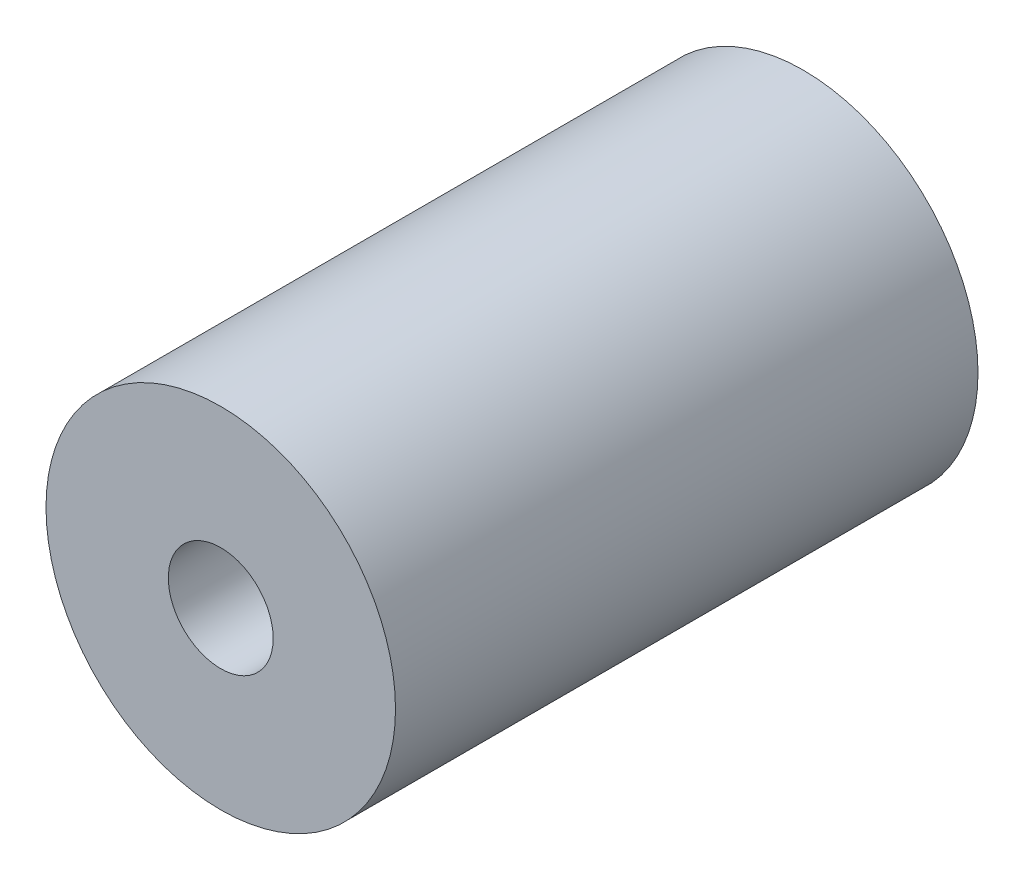
from build123d import *

# Parameters (mm, degrees)
SKETCH_1_R      = 15
SKETCH_1_R_2    = 4.5
EXTRUDE_1_DEPTH = 50


with BuildPart() as part:
    # 草图1 → 凸台-拉伸1 (new body)
    with BuildSketch(Plane.XY):
        Circle(SKETCH_1_R)
        Circle(SKETCH_1_R_2, mode=Mode.SUBTRACT)
    extrude(amount=EXTRUDE_1_DEPTH)


solid = part.part
